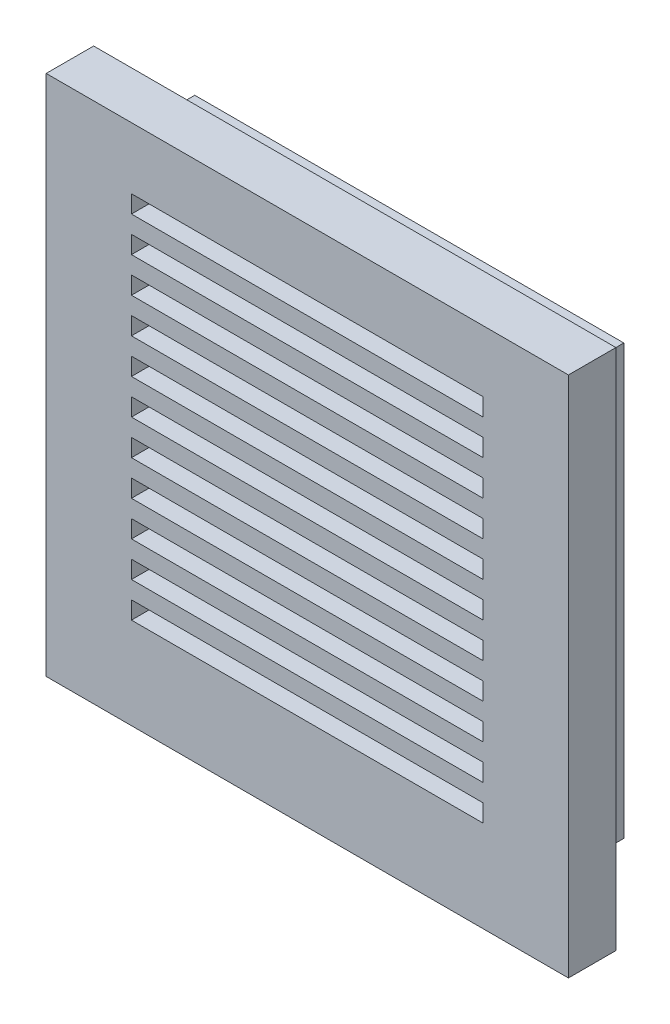
SolidWorks part; units mm, degrees
material "OTHER"
ref_plane "前视基准面" through (0, 0, 0) normal (0, 0, 1) x (1, 0, 0)
ref_plane "上视基准面" through (0, 0, 0) normal (0, 1, 0) x (1, 0, 0)
ref_plane "右视基准面" through (0, 0, 0) normal (1, 0, 0) x (0, 0, -1)
sketch "草图1" plane through (0, 0, 0) normal (0, 0, 1) x (1, 0, 0)
  line L1 (-61, 61) -> (61, 61)
  line L2 (-61, 61) -> (-61, -61)
  line L3 (-61, -61) -> (61, -61)
  line L4 (61, 61) -> (61, -61)
  line L5 (-61, 61) -> (61, -61) construction
  line L6 (-61, -61) -> (61, 61) construction
  point P0 (0, 0)
  dimension "D1" = 122
extrude "凸台-拉伸1" add sketch "草图1" along normal blind 15.5
sketch "草图2" plane through (0, 0, 15.5) normal (0, 0, 1) x (1, 0, 0)
  line L1 (-74.25, 74.25) -> (74.25, 74.25)
  line L2 (-74.25, 74.25) -> (-74.25, -74.25)
  line L3 (-74.25, -74.25) -> (74.25, -74.25)
  line L4 (74.25, 74.25) -> (74.25, -74.25)
  line L5 (-74.25, 74.25) -> (74.25, -74.25) construction
  line L6 (-74.25, -74.25) -> (74.25, 74.25) construction
  point P0 (0, 0)
  dimension "D1" = 148.5
extrude "凸台-拉伸2" add sketch "草图2" along normal blind 13.5
sketch "草图3" plane through (0, 0, 29) normal (0, 0, 1) x (1, 0, 0)
  line L0 (74.25, 74.25) -> (-74.25, 74.25) construction
  line L1 (-50, 56.75) -> (50, 56.75)
  line L2 (-50, 56.75) -> (-50, 51.75)
  line L3 (-50, 51.75) -> (50, 51.75)
  line L4 (50, 56.75) -> (50, 51.75)
  line L5 (-50, 56.75) -> (50, 51.75) construction
  line L6 (-50, 51.75) -> (50, 56.75) construction
  point P0 (0, 54.25)
  dimension "D1" = 5
  dimension "D2" = 100
  dimension "D3" = 20
extrude "切除-拉伸1" cut sketch "草图3" against normal through all
pattern_linear "阵列(线性)1" count 11 spacing 10 along (0, -1, 0) of "切除-拉伸1"
hole_wizard "大小mm 暗销孔1" positions "草图4" profile "草图5" hole size "Ø5.0" standard "ISO"
sketch "草图4" plane through (0, 0, 15.5) normal (0, 0, -1) x (-1, 0, 0)
  line L0 (0, 0) -> (0, 13.7182) construction
  line L2 (0, 0) -> (-30.5637, 0) construction
  point P0 (-65.5, 65.5)
  point P2 (0, 65.5)
  point P4 (65.5, 65.5)
  point P6 (65.5, 0)
  point P8 (-65.5, 0)
  point P10 (-65.5, -65.5)
  point P12 (0, -65.5)
  point P14 (65.5, -65.5)
  dimension "D1" = 131
  dimension "D2" = 131
sketch "草图5" plane through (65.5, 65.5, 15.5) normal (1, 0, 0) x (0, 1, 0)
  line L0 (0, 0) -> (0, 11.5022)
  line L1 (0, 11.5022) -> (2.5, 10)
  line L2 (2.5, 10) -> (2.5, 0)
  line L5 (2.5, 0) -> (0, 0)
  line L10 (0, 11.5022) -> (-2.5, 10) construction
  line L11 (0, -6.35) -> (0, 107.95) construction
  dimension "孔直径" = 5
  dimension "孔深度" = 10
  dimension "导头角度" = 118
hole_wizard "M4 螺纹孔1" positions "草图6" profile "草图7" tap size "M4" standard "ISO"
sketch "草图6" plane through (0, 0, 0) normal (0, 0, -1) x (-1, 0, 0)
  line L1 (0, 0) -> (-80.8896, 0) construction
  line L3 (0, 0) -> (0, -85.6427) construction
  point P0 (-52.5, 52.5)
  point P2 (52.5, 52.5)
  point P4 (52.5, -52.5)
  point P6 (-52.5, -52.5)
  dimension "D1" = 105
  dimension "D2" = 105
sketch "草图7" plane through (52.5, 52.5, 0) normal (1, 0, 0) x (0, 1, 0)
  line L0 (0, 0) -> (0, 11.0914)
  line L1 (0, 11.0914) -> (1.65, 10.1)
  line L2 (1.65, 10.1) -> (1.65, 0)
  line L5 (1.65, 0) -> (0, 0)
  line L10 (0, 11.0914) -> (-1.65, 10.1) construction
  line L11 (0, -6.35) -> (0, 107.95) construction
  dimension "螺纹孔钻头直径" = 3.3
  dimension "螺纹孔钻头深度" = 10.1
  dimension "导头角度" = 118
cosmetic thread "孔螺蚊线1" parameters "D1"=8, "D2"=4
cosmetic thread "孔螺蚊线2" parameters "D1"=8, "D2"=4
cosmetic thread "孔螺蚊线3" parameters "D1"=8, "D2"=4
cosmetic thread "孔螺蚊线4" parameters "D1"=8, "D2"=4
